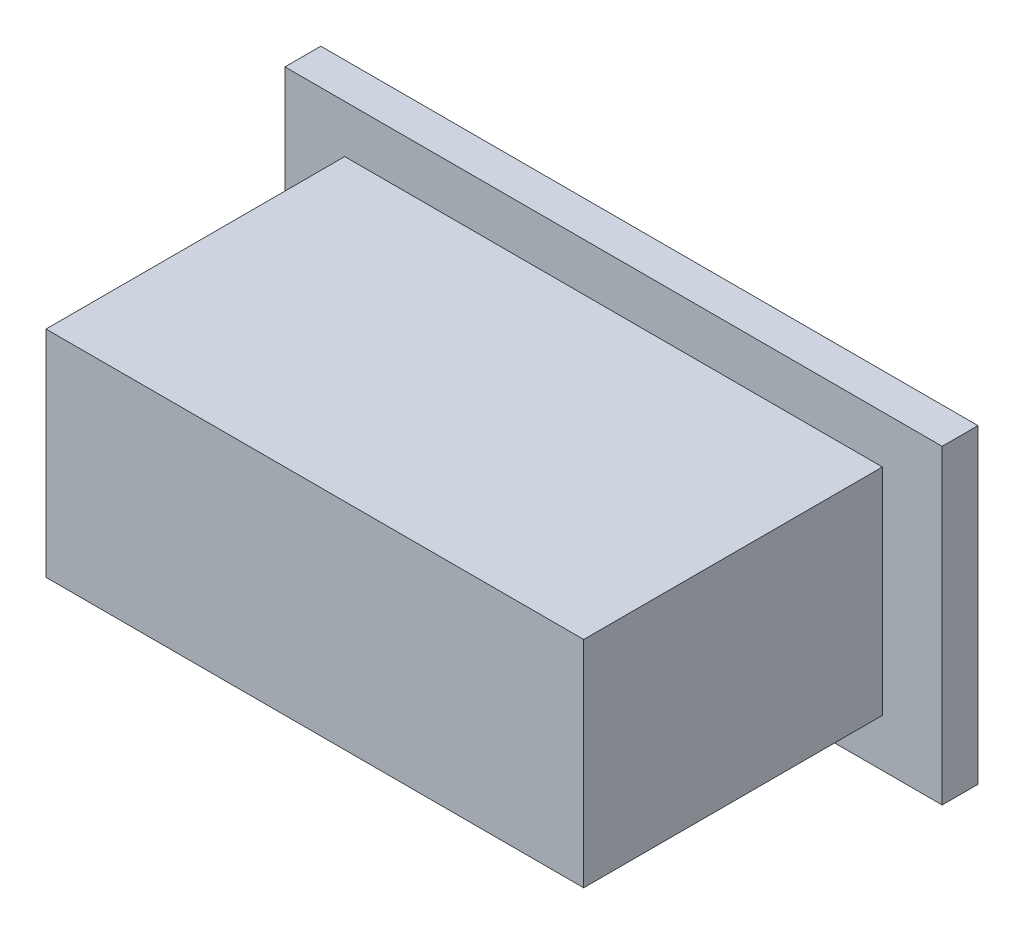
SolidWorks part; units mm, degrees
ref_plane "Front Plane" through (0, 0, 0) normal (0, 0, 1) x (1, 0, 0)
ref_plane "Top Plane" through (0, 0, 0) normal (0, 1, 0) x (1, 0, 0)
ref_plane "Right Plane" through (0, 0, 0) normal (1, 0, 0) x (0, 0, -1)
other "Configuration Table"
sketch "Sketch1" plane through (0, 0, 0) normal (0, 1, 0) x (1, 0, 0)
  line L0 (0, 0) -> (450, 0)
  line L1 (450, 0) -> (450, -280)
  line L2 (450, -280) -> (0, -280)
  line L3 (0, -280) -> (0, 0)
  dimension "D1" = 450
  dimension "D2" = 280
extrude "Boss-Extrude1" add sketch "Sketch1" along normal blind 180
sketch "Sketch2" plane through (0, 0, 0) normal (0, -1, 0) x (1, 0, 0)
  line L1 (-50, 30) -> (500, 30)
  line L2 (-50, 30) -> (-50, 0)
  line L3 (-50, 0) -> (500, 0)
  line L4 (500, 30) -> (500, 0)
  line L5 (0, 0) -> (0, 280) construction
  line L6 (450, 280) -> (450, 0) construction
  line L7 (450, 0) -> (0, 0) construction
  dimension "D1" = 30
  dimension "D2" = 50
  dimension "D3" = 50
extrude "Boss-Extrude2" add sketch "Sketch2" along normal blind 40 and the other way blind 220
